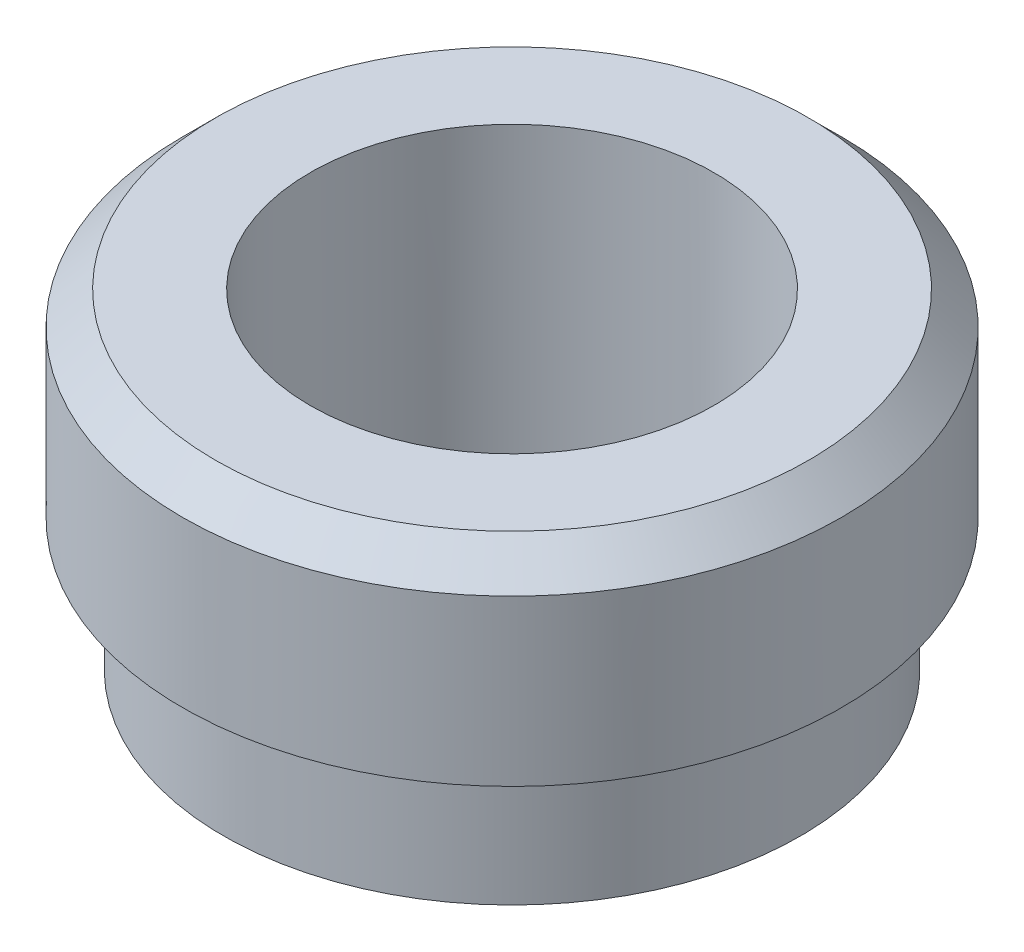
from build123d import *

# Parameters (mm, degrees)
G3_4_TAPPED_HOLE1_D     = 24.5
G3_4_TAPPED_HOLE1_DEPTH = 58.32
G3_4_TAPPED_HOLE1_TIP   = 7.360542583
CHAMFER1_SIZE           = 2


with BuildPart() as part:
    # Sketch1 → Revolve1 (revolve)
    with BuildSketch(Plane.XY, mode=Mode.PRIVATE) as revolve1_sk:
        Polygon((0, 0), (20, 0), (20, -12), (17.5, -12), (17.5, -20), (0, -20), align=None)
    revolve(revolve1_sk.sketch.rotate(Axis((0, -20, 0), (0, 1, 0)), 90), axis=Axis((0, -20, 0), (0, 1, 0)))

    # G3/4 Tapped Hole1
    with Locations(Plane(origin=(0, 0, 0), x_dir=(1, 0, 0), z_dir=(0, 1, 0))):
        with Locations((0, 0)):
            Hole(G3_4_TAPPED_HOLE1_D / 2, depth=G3_4_TAPPED_HOLE1_DEPTH)
            with Locations((0, 0, -(G3_4_TAPPED_HOLE1_DEPTH + G3_4_TAPPED_HOLE1_TIP / 2))):  # 118° drill point
                Cone(0, G3_4_TAPPED_HOLE1_D / 2, G3_4_TAPPED_HOLE1_TIP, mode=Mode.SUBTRACT)

    # Chamfer1
    chamfer1_edges = [part.edges().sort_by_distance(p)[0] for p in [
        (0, 0, 20),
    ]]
    chamfer(chamfer1_edges, length=CHAMFER1_SIZE)


solid = part.part
